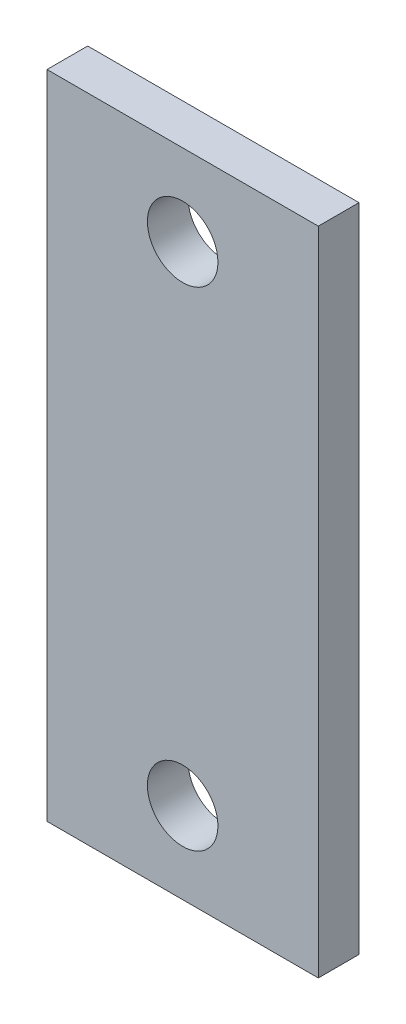
from build123d import *

# Parameters (mm, degrees)
SKETCH1_W           = 100
SKETCH1_H           = 240
BOSS_EXTRUDE1_DEPTH = 7.5
SKETCH2_R           = 13
CUT_EXTRUDE1_DEPTH  = 32


with BuildPart() as part:
    # Sketch1 → Boss-Extrude1 (new, symmetric)
    with BuildSketch(Plane.XY):
        Rectangle(SKETCH1_W, SKETCH1_H)
    extrude(amount=BOSS_EXTRUDE1_DEPTH, both=True)

    # Sketch2 → Cut-Extrude1 (cut)
    with BuildSketch(Plane.XY.offset(7.5)):
        with Locations((0, 90)):
            Circle(SKETCH2_R)
        with Locations((0, -90)):
            Circle(SKETCH2_R)
    extrude(amount=-CUT_EXTRUDE1_DEPTH, mode=Mode.SUBTRACT)


solid = part.part
